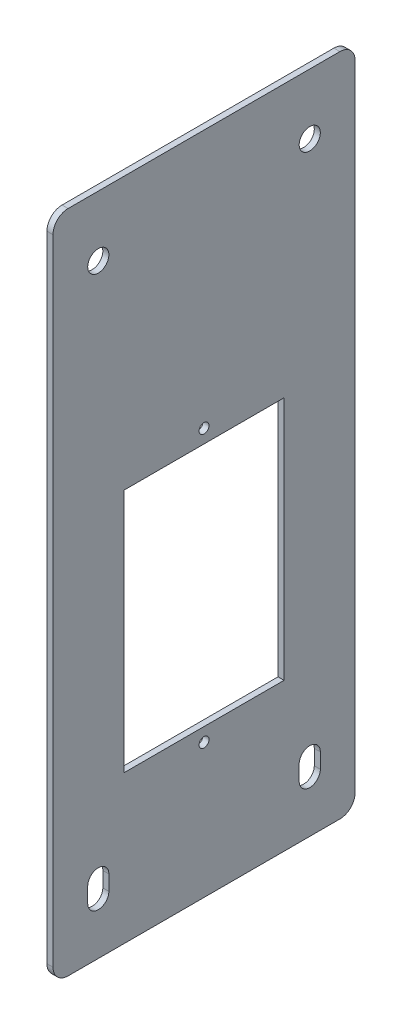
from build123d import *

# Parameters (mm, degrees)
SKETCH_1_W          = 2
SKETCH_1_H          = 220
EXTRUDE_1_DEPTH     = 100
SKETCH_2_R          = 1.65
SKETCH_2_R_2        = 3.5
SKETCH_2_W          = 53
SKETCH_2_H          = 81
CUT_EXTRUDE_1_DEPTH = 10
FILLET_1_R          = 5


with BuildPart() as part:
    # 草图1 → 拉伸-薄壁1 (new body)
    with BuildSketch(Plane.XY):
        with Locations((1, 110)):
            Rectangle(SKETCH_1_W, SKETCH_1_H)
    extrude(amount=-EXTRUDE_1_DEPTH)

    # 草图2 → 切除-拉伸1 (cut)
    with BuildSketch(Plane.ZY):
        with Locations(Location((-50, 44.5, 0), (0, 0, 270))):
            Circle(SKETCH_2_R)
        with Locations(Location((-50, 134.5, 0), (0, 0, 270))):
            Circle(SKETCH_2_R)
        with Locations(Location((-15, 200, 0), (0, 0, 270))):
            Circle(SKETCH_2_R_2)
        with Locations(Location((-85, 200, 0), (0, 0, 270))):
            Circle(SKETCH_2_R_2)
        with Locations((-50, 89.5)):
            Rectangle(SKETCH_2_W, SKETCH_2_H)
        with BuildLine():
            Line((-11.5, 22.5), (-11.5, 17.5))
            ThreePointArc((-11.5, 17.5), (-15, 14), (-18.5, 17.5))
            Line((-18.5, 17.5), (-18.5, 22.5))
            ThreePointArc((-18.5, 22.5), (-15, 26), (-11.5, 22.5))
        make_face()
        with BuildLine():
            Line((-81.5, 22.5), (-81.5, 17.5))
            ThreePointArc((-81.5, 17.5), (-85, 14), (-88.5, 17.5))
            Line((-88.5, 17.5), (-88.5, 22.5))
            ThreePointArc((-88.5, 22.5), (-85, 26), (-81.5, 22.5))
        make_face()
    extrude(amount=-CUT_EXTRUDE_1_DEPTH, mode=Mode.SUBTRACT)

    # 圆角1
    fillet_1_edges = [part.edges().sort_by_distance(p)[0] for p in [
        (1, 220, -100),
        (1, 220, 0),
        (1, 0, 0),
        (1, 0, -100),
    ]]
    fillet(fillet_1_edges, radius=FILLET_1_R)


solid = part.part
